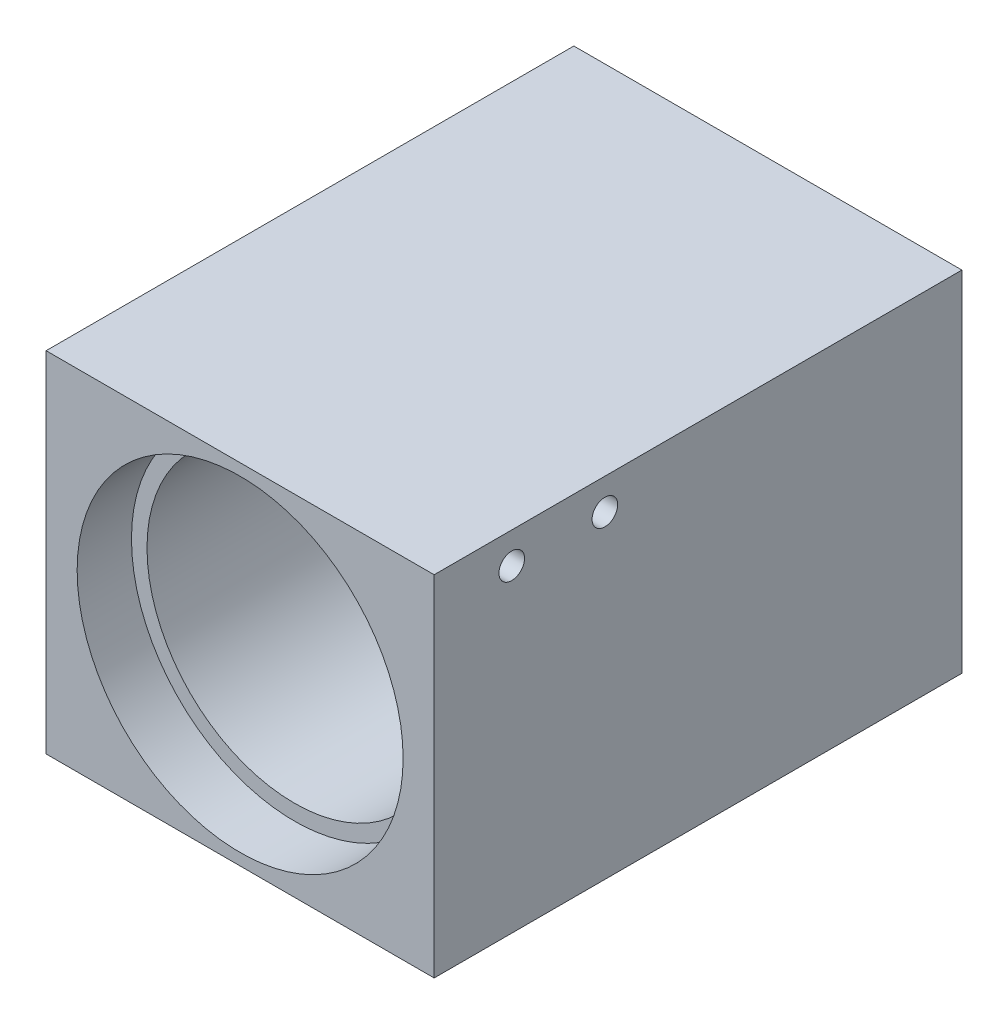
SolidWorks part; units mm, degrees
ref_plane "前视基准面" through (0, 0, 0) normal (0, 0, 1) x (1, 0, 0)
ref_plane "上视基准面" through (0, 0, 0) normal (0, 1, 0) x (1, 0, 0)
ref_plane "右视基准面" through (0, 0, 0) normal (1, 0, 0) x (0, 0, -1)
sketch "草图1" plane through (0, 0, 0) normal (0, 0, 1) x (1, 0, 0)
  line L1 (0, 0) -> (50, 0)
  line L2 (0, 0) -> (0, 45)
  line L3 (0, 45) -> (50, 45)
  line L4 (50, 0) -> (50, 45)
  dimension "D1" = 50
  dimension "D2" = 45
extrude "凸台-拉伸1" add sketch "草图1" along normal blind 68
sketch "草图2" plane through (0, 0, 0) normal (0, 0, -1) x (-1, 0, 0)
  line L0 (-25, 45) -> (-25, 0) construction
  line L1 (-50, 45) -> (0, 45) construction
  line L2 (0, 0) -> (-50, 0) construction
  circle A0 centre (-25, 22.5) radius 19
  dimension "D1" = 38
extrude "切除-拉伸1" cut sketch "草图2" against normal blind 79
sketch "草图3" plane through (0, 0, 68) normal (0, 0, 1) x (1, 0, 0)
  circle A0 centre (25, 22.5) radius 21
  dimension "D1" = 42
extrude "切除-拉伸2" cut sketch "草图3" against normal blind 7
sketch "草图4" plane through (0, 0, 0) normal (0, 0, -1) x (-1, 0, 0)
  circle A0 centre (-25, 22.5) radius 21
  dimension "D1" = 42
extrude "切除-拉伸3" cut sketch "草图4" against normal blind 25
hole_wizard "M4 螺纹孔1" positions "草图6" profile "草图5" tap size "M4" standard "GB"
sketch "草图6" plane through (50, 0, 0) normal (1, 0, 0) x (0, 0, -1)
  line L0 (-68, 0) -> (-68, 45) construction
  line L1 (-68, 45) -> (0, 45) construction
  point P0 (-58, 41)
  point P3 (-46, 41)
  dimension "D1" = 12
  dimension "D2" = 10
  dimension "D3" = 4
sketch "草图5" plane through (50, 41, 58) normal (0, 1, 0) x (0, 0, -1)
  line L0 (0, 0) -> (0, 11.0914)
  line L1 (0, 11.0914) -> (1.65, 10.1)
  line L2 (1.65, 10.1) -> (1.65, 0)
  line L5 (1.65, 0) -> (0, 0)
  line L10 (0, 11.0914) -> (-1.65, 10.1) construction
  line L11 (0, -6.35) -> (0, 107.95) construction
  dimension "螺纹孔钻头直径" = 3.3
  dimension "螺纹孔钻头深度" = 10.1
  dimension "导头角度" = 118
cosmetic thread "孔螺蚊线2" parameters "D1"=8, "D2"=4
cosmetic thread "孔螺蚊线13" parameters "D1"=8, "D2"=4
hole_wizard "M4 螺纹孔2" positions "草图8" profile "草图7" tap size "M4" standard "GB"
sketch "草图8" plane through (0, 0, 0) normal (-1, 0, 0) x (0, 0, 1)
  circle A0 centre (46, 41) radius 1.65 construction
  circle A1 centre (58, 41) radius 1.65 construction
  point P0 (46, 41)
  point P3 (58, 41)
sketch "草图7" plane through (0, 41, 46) normal (0, 1, 0) x (0, 0, 1)
  line L0 (0, 0) -> (0, 11.0914)
  line L1 (0, 11.0914) -> (1.65, 10.1)
  line L2 (1.65, 10.1) -> (1.65, 0)
  line L5 (1.65, 0) -> (0, 0)
  line L10 (0, 11.0914) -> (-1.65, 10.1) construction
  line L11 (0, -6.35) -> (0, 107.95) construction
  dimension "螺纹孔钻头直径" = 3.3
  dimension "螺纹孔钻头深度" = 10.1
  dimension "导头角度" = 118
cosmetic thread "孔螺蚊线3" parameters "D1"=8, "D2"=4
cosmetic thread "孔螺蚊线14" parameters "D1"=8, "D2"=4
hole_wizard "Ø6.5 (6.5) 直径孔1" positions "草图12" profile "草图11" hole size "Ø6.5" standard "GB"
sketch "草图12" plane through (0, 0, 0) normal (0, -1, 0) x (-1, 0, 0)
  line L0 (-25, -68) -> (-25, 0) construction
  line L1 (0, -68) -> (-50, -68) construction
  line L2 (0, 0) -> (-50, 0) construction
  point P0 (-25, -38)
  dimension "D1" = 30
sketch "草图11" plane through (25, 0, 38) normal (1, 0, 0) x (0, 0, -1)
  line L0 (0, 0) -> (0, 21.9528)
  line L1 (0, 21.9528) -> (3.25, 20)
  line L2 (3.25, 20) -> (3.25, 0)
  line L5 (3.25, 0) -> (0, 0)
  line L10 (0, 21.9528) -> (-3.25, 20) construction
  line L11 (0, -6.35) -> (0, 107.95) construction
  dimension "孔直径" = 6.5
  dimension "孔深度" = 20
  dimension "导头角度" = 118
hole_wizard "M4 螺纹孔4" positions "草图16" profile "草图15" tap size "M4" standard "GB"
sketch "草图16" plane through (0, 0, 0) normal (0, 0, -1) x (-1, 0, 0)
  line L0 (-25, 45) -> (-25, 0) construction
  line L1 (-50, 45) -> (0, 45) construction
  line L2 (0, 0) -> (-50, 0) construction
  line L4 (0, 22.5) -> (-50, 22.5) construction
  line L5 (0, 45) -> (0, 0) construction
  line L6 (-50, 0) -> (-50, 45) construction
  point P0 (-5, 36.5)
  point P2 (-45, 36.5)
  point P4 (-45, 8.5)
  point P6 (-5, 8.5)
  dimension "D1" = 28
  dimension "D2" = 40
sketch "草图15" plane through (5, 36.5, 0) normal (1, 0, 0) x (0, 1, 0)
  line L0 (0, 0) -> (0, 11.0914)
  line L1 (0, 11.0914) -> (1.65, 10.1)
  line L2 (1.65, 10.1) -> (1.65, 0)
  line L5 (1.65, 0) -> (0, 0)
  line L10 (0, 11.0914) -> (-1.65, 10.1) construction
  line L11 (0, -6.35) -> (0, 107.95) construction
  dimension "螺纹孔钻头直径" = 3.3
  dimension "螺纹孔钻头深度" = 10.1
  dimension "导头角度" = 118
cosmetic thread "孔螺蚊线7" parameters "D1"=8, "D2"=4
cosmetic thread "孔螺蚊线8" parameters "D1"=8, "D2"=4
cosmetic thread "孔螺蚊线9" parameters "D1"=8, "D2"=4
cosmetic thread "孔螺蚊线10" parameters "D1"=8, "D2"=4
